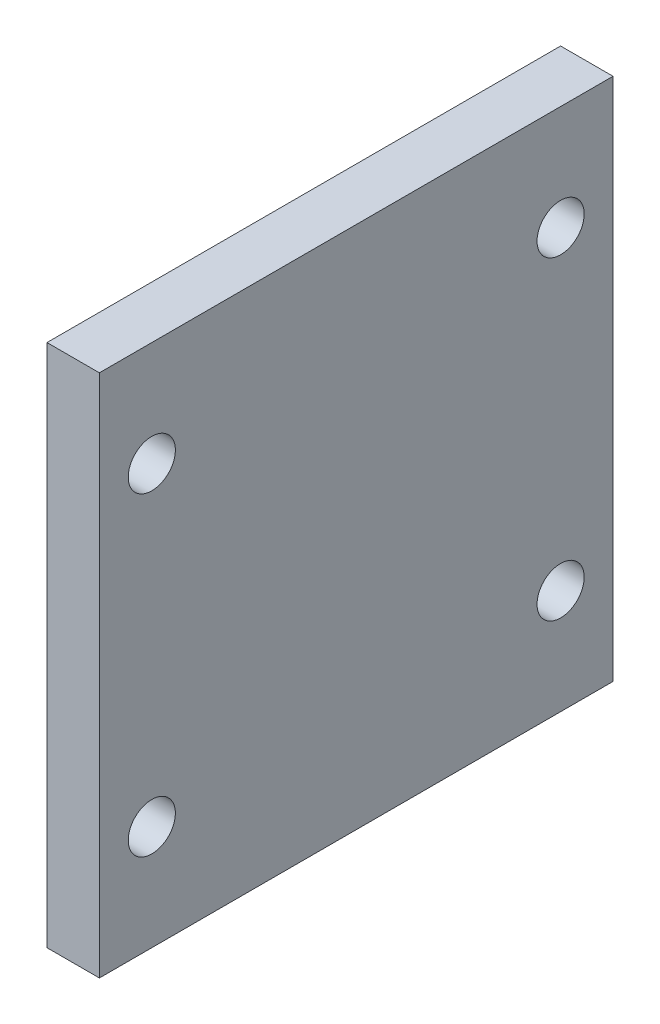
from build123d import *

# Parameters (mm, degrees)
SKETCH_1_W            = 98
SKETCH_1_H            = 100
EXTRUDE_1_DEPTH       = 10
HOLE_WIZARD_9_0_9_1_D = 9


with BuildPart() as part:
    # 草图1 → 凸台-拉伸1 (new body)
    with BuildSketch(Plane(origin=(0, 0, 0), x_dir=(0, 0, -1), z_dir=(1, 0, 0))):
        Rectangle(SKETCH_1_W, SKETCH_1_H)
    extrude(amount=EXTRUDE_1_DEPTH)

    # Ø9.0 (9) 直径孔1 (through all)
    with Locations(Plane(origin=(10, 0, 0), x_dir=(0, 0, -1), z_dir=(1, 0, 0))):
        with Locations((-39, 30), (39, 30), (-39, -30), (39, -30)):
            Hole(HOLE_WIZARD_9_0_9_1_D / 2)


solid = part.part
